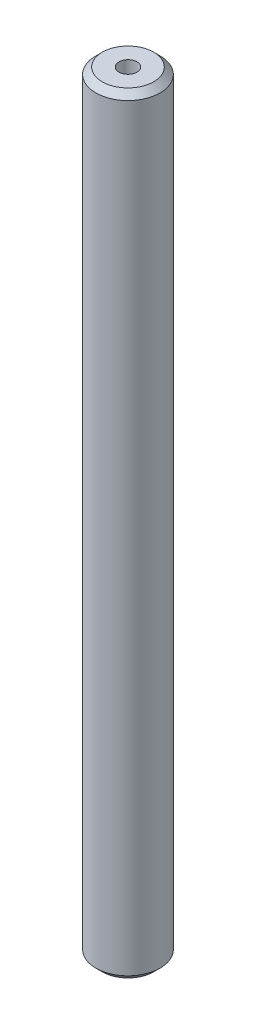
from build123d import *

# Parameters (mm, degrees)
SKETCH1_R              = 25
BOSS_EXTRUDE1_DEPTH    = 600
CHAMFER1_SIZE          = 5
M16_TAPPED_HOLE1_D     = 14
M16_TAPPED_HOLE1_DEPTH = 38
M16_TAPPED_HOLE1_TIP   = 4.206024333
M16_TAPPED_HOLE2_D     = 14
M16_TAPPED_HOLE2_DEPTH = 38
M16_TAPPED_HOLE2_TIP   = 4.206024333


with BuildPart() as part:
    # Sketch1 → Boss-Extrude1 (new body)
    with BuildSketch(Plane(origin=(0, 0, 0), x_dir=(1, 0, 0), z_dir=(0, 1, 0))):
        with Locations(Location((0, 0, 0), (0, 0, 270))):
            Circle(SKETCH1_R)
    extrude(amount=BOSS_EXTRUDE1_DEPTH)

    # Chamfer1
    chamfer1_edges = [part.edges().sort_by_distance(p)[0] for p in [
        (0, 0, -25),
        (0, 600, -25),
    ]]
    chamfer(chamfer1_edges, length=CHAMFER1_SIZE)

    # M16 Tapped Hole1
    with Locations(Plane(origin=(0, 600, 0), x_dir=(1, 0, 0), z_dir=(0, 1, 0))):
        with Locations((0, 0)):
            Hole(M16_TAPPED_HOLE1_D / 2, depth=M16_TAPPED_HOLE1_DEPTH)
            with Locations((0, 0, -(M16_TAPPED_HOLE1_DEPTH + M16_TAPPED_HOLE1_TIP / 2))):  # 118° drill point
                Cone(0, M16_TAPPED_HOLE1_D / 2, M16_TAPPED_HOLE1_TIP, mode=Mode.SUBTRACT)

    # M16 Tapped Hole2
    with Locations(Plane(origin=(0, 0, 0), x_dir=(-1, 0, 0), z_dir=(0, -1, 0))):
        with Locations((0, 0)):
            Hole(M16_TAPPED_HOLE2_D / 2, depth=M16_TAPPED_HOLE2_DEPTH)
            with Locations((0, 0, -(M16_TAPPED_HOLE2_DEPTH + M16_TAPPED_HOLE2_TIP / 2))):  # 118° drill point
                Cone(0, M16_TAPPED_HOLE2_D / 2, M16_TAPPED_HOLE2_TIP, mode=Mode.SUBTRACT)


solid = part.part
